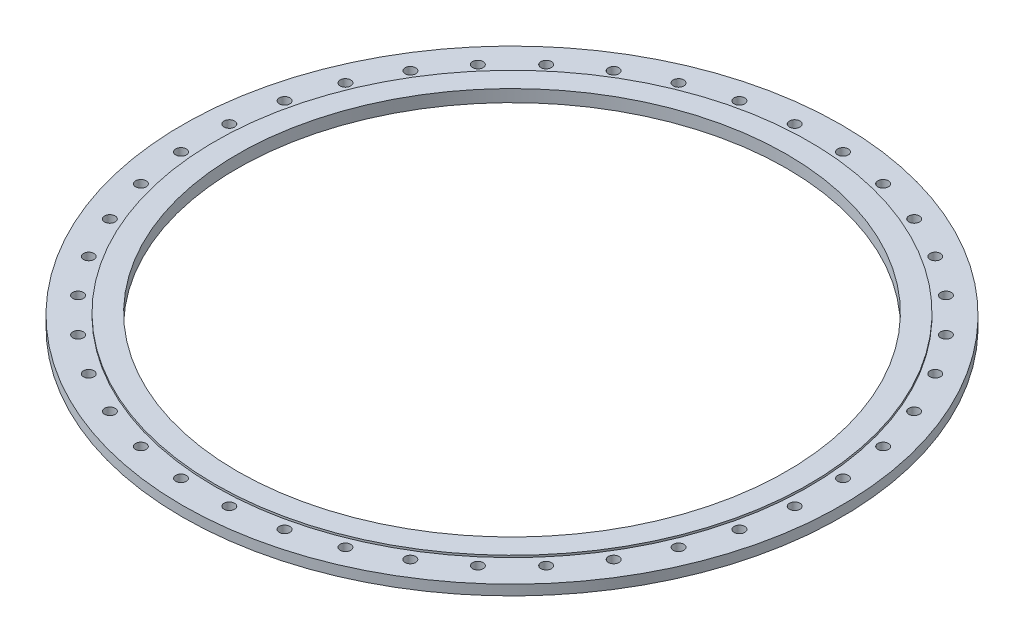
from build123d import *

# Parameters (mm, degrees)
SKETCH_1_R                = 810
EXTRUDE_1_DEPTH           = 25
SKETCH_2_R                = 730
EXTRUDE_2_DEPTH           = 5
CUT_EXTRUDE_1_REACH       = 1147.906
SKETCH_3_R                = 75
SKETCH_4_R                = 110
CUT_EXTRUDE_2_DEPTH       = 5
HOLE_WIZARD_M8_1_D        = 6.8
HOLE_WIZARD_25_5_25_5_1_D = 26
CUT_EXTRUDE_3_DEPTH       = 1146.905755287
CUT_EXTRUDE_3_DEPTH_BACK  = 1146.905755287
SKETCH_10_R               = 675


with BuildPart() as part:
    # 草图1 → 凸台-拉伸1 (new body)
    with BuildSketch(Plane(origin=(0, 0, 0), x_dir=(1, 0, 0), z_dir=(0, 1, 0))):
        with Locations(Location((0, 0, 0), (0, 0, 270))):
            Circle(SKETCH_1_R)
    extrude(amount=EXTRUDE_1_DEPTH)

    # 草图2 → 凸台-拉伸2 (add)
    with BuildSketch(Plane(origin=(0, 25, 0), x_dir=(1, 0, 0), z_dir=(0, 1, 0))):
        with Locations(Location((0, 0, 0), (0, 0, 270))):
            Circle(SKETCH_2_R)
    extrude(amount=EXTRUDE_2_DEPTH)

    # 草图3 → 切除-拉伸1 (cut, up to next)
    with BuildSketch(Plane(origin=(0, 30, 0), x_dir=(1, 0, 0), z_dir=(0, 1, 0)), mode=Mode.PRIVATE) as cut_extrude_1_sk1:
        with BuildLine():
            Line((130, 662.363193422), (130, -662.363193422))
            ThreePointArc((130, -662.363193422), (521.236510617, -428.879353665), (675, 0))
            ThreePointArc((675, 0), (521.236510617, 428.879353665), (130, 662.363193422))
        make_face()
    cut_extrude_1_tool1 = extrude(cut_extrude_1_sk1.sketch, amount=-CUT_EXTRUDE_1_REACH, mode=Mode.PRIVATE) & part.part
    # 草图3 → 切除-拉伸1 (cut, up to next)
    with BuildSketch(Plane(origin=(0, 30, 0), x_dir=(1, 0, 0), z_dir=(0, 1, 0)), mode=Mode.PRIVATE) as cut_extrude_1_sk2:
        with BuildLine():
            ThreePointArc((-130, 662.363193422), (-675, 0), (-130, -662.363193422))
            Line((-130, -662.363193422), (-130, 662.363193422))
        make_face()
    cut_extrude_1_tool2 = extrude(cut_extrude_1_sk2.sketch, amount=-CUT_EXTRUDE_1_REACH, mode=Mode.PRIVATE) & part.part
    # 草图3 → 切除-拉伸1 (cut, up to next)
    with BuildSketch(Plane(origin=(0, 30, 0), x_dir=(1, 0, 0), z_dir=(0, 1, 0)), mode=Mode.PRIVATE) as cut_extrude_1_sk3:
        with Locations(Location((0, 0, 0), (0, 0, 270))):
            Circle(SKETCH_3_R)
    cut_extrude_1_tool3 = extrude(cut_extrude_1_sk3.sketch, amount=-CUT_EXTRUDE_1_REACH, mode=Mode.PRIVATE) & part.part
    add(cut_extrude_1_tool1.solids().sort_by_distance((357.907844, 30, 0))[0], mode=Mode.SUBTRACT)
    add(cut_extrude_1_tool2.solids().sort_by_distance((-357.907844, 30, 0))[0], mode=Mode.SUBTRACT)
    add(cut_extrude_1_tool3.solids().sort_by_distance((0, 30, 0))[0], mode=Mode.SUBTRACT)

    # 草图4 → 切除-拉伸2 (cut)
    with BuildSketch(Plane(origin=(0, 30, 0), x_dir=(1, 0, 0), z_dir=(0, 1, 0))):
        with Locations(Location((0, 0, 0), (0, 0, 270))):
            Circle(SKETCH_4_R)
    extrude(amount=-CUT_EXTRUDE_2_DEPTH, mode=Mode.SUBTRACT)

    # M8 螺纹孔1 (through all)
    with Locations(Plane(origin=(0, 25, 0), x_dir=(1, 0, 0), z_dir=(0, 1, 0))):
        with Locations((0, 85), (85, 0), (0, -85), (-85, 0)):
            Hole(HOLE_WIZARD_M8_1_D / 2)

    # Ø25.5 (25.5) 直径孔1 (through all)
    with Locations(Plane(origin=(0, 25, 0), x_dir=(1, 0, 0), z_dir=(0, 1, 0))):
        with Locations((-59.354305918, 754.167962969), (59.354305918, 754.167962969), (176.601417757, 735.597844781), (289.500016584, 698.914866345), (395.270164208, 645.022284334), (491.307448562, 575.247112976), (575.247112976, 491.307448562), (645.022284334, 395.270164208), (698.914866345, 289.500016584), (735.597844781, 176.601417757), (754.167962969, 59.354305918), (754.167962969, -59.354305918), (735.597844781, -176.601417757), (698.914866345, -289.500016584), (645.022284334, -395.270164208), (575.247112976, -491.307448562), (491.307448562, -575.247112976), (395.270164208, -645.022284334), (289.500016584, -698.914866345), (176.601417757, -735.597844781), (59.354305918, -754.167962969), (-59.354305918, -754.167962969), (-176.601417757, -735.597844781), (-289.500016584, -698.914866345), (-395.270164208, -645.022284334), (-491.307448562, -575.247112976), (-575.247112976, -491.307448562), (-645.022284334, -395.270164208), (-698.914866345, -289.500016584), (-735.597844781, -176.601417757), (-754.167962969, -59.354305918), (-754.167962969, 59.354305918), (-735.597844781, 176.601417757), (-698.914866345, 289.500016584), (-645.022284334, 395.270164208), (-575.247112976, 491.307448562), (-491.307448562, 575.247112976), (-395.270164208, 645.022284334), (-289.500016584, 698.914866345), (-176.601417757, 735.597844781)):
            Hole(HOLE_WIZARD_25_5_25_5_1_D / 2)

    # 草图10 → 切除-拉伸3 (cut, two sides: drawn at the far end of the back side and taken through both)
    with BuildSketch(Plane(origin=(0, 30, 0), x_dir=(1, 0, 0), z_dir=(0, 1, 0)).offset(-CUT_EXTRUDE_3_DEPTH_BACK)):
        with Locations(Location((0, 0, 0), (0, 0, 270))):
            Circle(SKETCH_10_R)
    extrude(amount=CUT_EXTRUDE_3_DEPTH + CUT_EXTRUDE_3_DEPTH_BACK, mode=Mode.SUBTRACT)


solid = part.part
